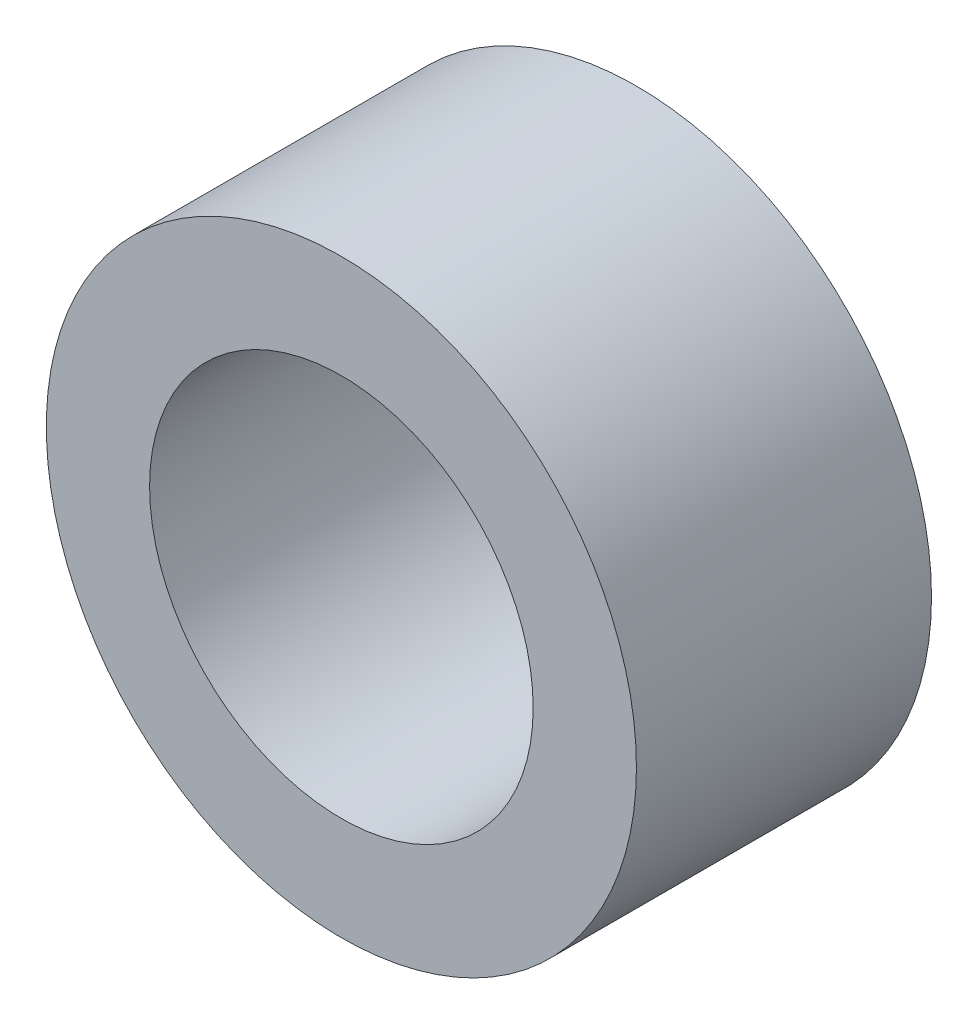
SolidWorks part; units mm, degrees
ref_plane "Front Plane" through (0, 0, 0) normal (0, 0, 1) x (1, 0, 0)
ref_plane "Top Plane" through (0, 0, 0) normal (0, 1, 0) x (1, 0, 0)
ref_plane "Right Plane" through (0, 0, 0) normal (1, 0, 0) x (0, 0, -1)
sketch "Sketch1" plane through (0, 0, 0) normal (0, 0, 1) x (1, 0, 0)
  circle A0 centre (0, 0) radius 10
  dimension "D1" = 20
extrude "Extrude1" add sketch "Sketch1" along normal blind 10
sketch "Sketch2" plane through (0, 0, 10) normal (0, 0, 1) x (1, 0, 0)
  circle A0 centre (0, 0) radius 6.5
  dimension "D1" = 13
extrude "Cut-Extrude1" cut sketch "Sketch2" against normal blind 10
